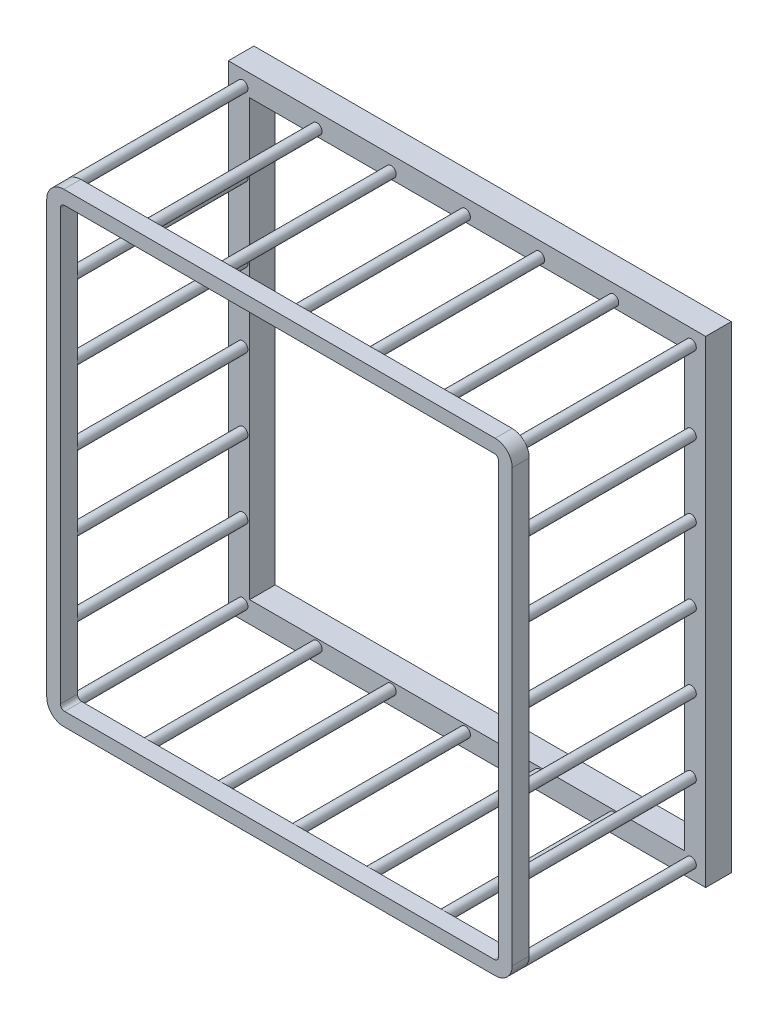
SolidWorks part; units mm, degrees
ref_plane "Front Plane" through (0, 0, 0) normal (0, 0, 1) x (1, 0, 0)
ref_plane "Top Plane" through (0, 0, 0) normal (0, 1, 0) x (1, 0, 0)
ref_plane "Right Plane" through (0, 0, 0) normal (1, 0, 0) x (0, 0, -1)
other "Configuration Table"
sketch "Sketch1" plane through (0, 0, 0) normal (0, 0, 1) x (1, 0, 0)
  line L0 (25, 535) -> (535, 535)
  line L1 (0, 0) -> (560, 0)
  line L2 (0, 0) -> (0, 560)
  line L3 (0, 560) -> (560, 560)
  line L4 (560, 0) -> (560, 560)
  line L5 (535, 25) -> (535, 535)
  line L6 (25, 25) -> (535, 25)
  line L7 (25, 25) -> (25, 535)
  dimension "D1" = 560
  dimension "D2" = 560
  dimension "D3" = 25
extrude "Boss-Extrude1" add sketch "Sketch1" along normal blind 30
sketch "Sketch2" plane through (0, 0, 30) normal (0, 0, 1) x (1, 0, 0)
  line L0 (25, 25) -> (535, 25) construction
  line L1 (17, 543) -> (543, 543) construction
  line L2 (17, 543) -> (17, 17) construction
  line L3 (17, 17) -> (543, 17) construction
  line L4 (543, 543) -> (543, 17) construction
  line L6 (535, 25) -> (535, 535) construction
  line L7 (535, 535) -> (25, 535) construction
  line L8 (25, 535) -> (25, 25) construction
  circle A0 centre (17, 543) radius 6
  circle A1 centre (17, 17) radius 6
  circle A2 centre (543, 17) radius 6
  circle A3 centre (543, 543) radius 6
  circle A4 centre (104, 543) radius 6
  circle A5 centre (104, 17) radius 6
  circle A6 centre (191, 543) radius 6
  circle A7 centre (191, 17) radius 6
  circle A8 centre (278, 543) radius 6
  circle A9 centre (278, 17) radius 6
  circle A10 centre (365, 543) radius 6
  circle A11 centre (365, 17) radius 6
  circle A12 centre (452, 543) radius 6
  circle A13 centre (452, 17) radius 6
  circle A14 centre (17, 104) radius 6
  circle A15 centre (543, 104) radius 6
  circle A16 centre (17, 191) radius 6
  circle A17 centre (543, 191) radius 6
  circle A18 centre (17, 278) radius 6
  circle A19 centre (543, 278) radius 6
  circle A20 centre (17, 365) radius 6
  circle A21 centre (543, 365) radius 6
  circle A22 centre (17, 452) radius 6
  circle A23 centre (543, 452) radius 6
  circle A26 centre (17, 539) radius 6 [skipped]
  circle A27 centre (543, 539) radius 6 [skipped]
  dimension "D5" = 12
  dimension "D1" = 8
  dimension "D2" = 8
  dimension "D3" = 8
  dimension "D4" = 8
  dimension "D6" = 6
  dimension "D7" = 7
extrude "Boss-Extrude2" add sketch "Sketch2" along normal blind 200
sketch "Sketch3" plane through (0, 0, 230) normal (0, 0, 1) x (1, 0, 0)
  line L0 (7, 533) -> (7, 27)
  line L1 (11, 549) -> (549, 549) construction
  line L2 (11, 549) -> (11, 11) construction
  line L3 (11, 11) -> (549, 11) construction
  line L4 (549, 549) -> (549, 11) construction
  line L5 (27, 7) -> (533, 7)
  line L6 (553, 533) -> (553, 27)
  line L7 (27, 553) -> (533, 553)
  line L8 (7, 553) -> (7, 7) construction
  line L9 (23, 532) -> (23, 28)
  line L10 (28, 23) -> (532, 23)
  line L11 (537, 532) -> (537, 28)
  line L12 (28, 537) -> (532, 537)
  line L13 (7, 553) -> (553, 553) construction
  line L14 (7, 7) -> (553, 7) construction
  line L15 (553, 553) -> (553, 7) construction
  line L16 (23, 537) -> (23, 23) construction
  line L17 (23, 23) -> (537, 23) construction
  line L18 (537, 537) -> (537, 23) construction
  line L19 (23, 537) -> (537, 537) construction
  arc A0 (7, 533) -> (27, 553) centre (27, 533) cw
  arc A1 (7, 27) -> (27, 7) centre (27, 27) ccw
  arc A2 (533, 7) -> (553, 27) centre (533, 27) ccw
  arc A3 (553, 533) -> (533, 553) centre (533, 533) ccw
  arc A4 (23, 28) -> (28, 23) centre (28, 28) ccw
  arc A5 (532, 23) -> (537, 28) centre (532, 28) ccw
  arc A6 (537, 532) -> (532, 537) centre (532, 532) ccw
  arc A7 (23, 532) -> (28, 537) centre (28, 532) cw
  dimension "D2" = 20
  dimension "D4" = 20
  dimension "D5" = 5
  dimension "D1" = 4
  dimension "D3" = 16
extrude "Boss-Extrude3" add sketch "Sketch3" along normal blind 20
